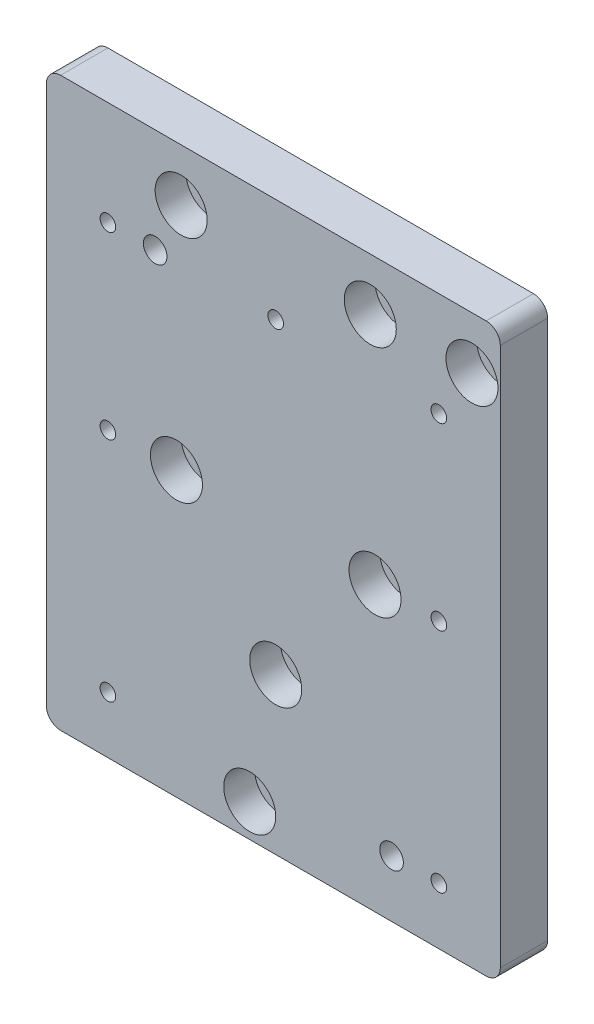
SolidWorks part; units mm, degrees
material "6061铝"
ref_plane "前视基准面" through (0, 0, 0) normal (0, 0, 1) x (1, 0, 0)
ref_plane "上视基准面" through (0, 0, 0) normal (0, 1, 0) x (1, 0, 0)
ref_plane "右视基准面" through (0, 0, 0) normal (1, 0, 0) x (0, 0, -1)
sketch "草图1" plane through (0, 0, 0) normal (0, 0, 1) x (1, 0, 0)
  line L1 (-48, 60) -> (48, 60)
  line L2 (-48, 60) -> (-48, -60)
  line L3 (-48, -60) -> (48, -60)
  line L4 (48, 60) -> (48, -60)
  line L5 (-48, 60) -> (48, -60) construction
  line L6 (-48, -60) -> (48, 60) construction
  point P0 (0, 0)
  dimension "D1" = 96
  dimension "D2" = 120
extrude "凸台-拉伸1" add sketch "草图1" along normal blind 10
hole_wizard "打孔尺寸(%根据)内六角圆柱头螺钉的类型2" positions "草图2" profile "草图4" counterbore size "M6" standard "GB" end condition through all
sketch "草图2" plane through (0, 0, 10) normal (0, 0, 1) x (1, 0, 0)
  point P0 (-19.5, 48.95)
  point P3 (20.5, 48.95)
  point P6 (42, 48.95)
  point P9 (21.5, -0.05)
  point P12 (-20.5, -0.05)
  point P15 (0.5, -27.05)
  point P18 (-5, -53.05)
sketch "草图4" plane through (-19.5, 48.95, 10) normal (1, 0, 0) x (0, -1, 0)
  line L0 (0, 0) -> (0, 10)
  line L1 (0, 10) -> (3.2, 10)
  line L3 (3.2, 10) -> (3.2, 6.5)
  line L4 (3.2, 6.5) -> (5.5, 6.5)
  line L5 (5.5, 6.5) -> (5.5, 0)
  line L7 (5.5, 0) -> (0, 0)
  line L11 (0, -6.35) -> (0, 107.95) construction
  dimension "通孔孔直径" = 6.4
  dimension "通孔孔深度" = 10
  dimension "柱形沉头孔直径" = 11
  dimension "柱形沉头孔深度" = 6.5
fillet "圆角1" radius 3 4 edges at (48, 60, 5) (-48, 60, 5) (-48, -60, 5) (48, -60, 5)
hole_wizard "M4 螺纹孔1" positions "草图5" profile "草图6" tap size "M4" standard "GB" end condition through all
sketch "草图5" plane through (0, 0, 10) normal (0, 0, 1) x (1, 0, 0)
  line L0 (0, 0) -> (0, -66.745) construction
  line L1 (-45, -60) -> (45, -60) construction
  line L2 (0.5, -27.05) -> (0.5, 29.2918) construction
  point P0 (-35, -48)
  point P6 (-35, 0)
  point P13 (35, 0)
  point P14 (35, -48)
  point P15 (-35, 38)
  point P23 (35, 38)
  point P26 (0.5, 38)
  point P47 (0, 0)
  point P48 (0, 0)
  dimension "D1" = 70
  dimension "D2" = 48
  dimension "D3" = 12
  dimension "D4" = 38
sketch "草图6" plane through (-35, -48, 10) normal (1, 0, 0) x (0, -1, 0)
  line L0 (0, 0) -> (0, 10)
  line L1 (0, 10) -> (1.65, 10)
  line L2 (1.65, 10) -> (1.65, 0)
  line L5 (1.65, 0) -> (0, 0)
  line L11 (0, -6.35) -> (0, 107.95) construction
  dimension "通孔螺纹孔钻头直径" = 3.3
  dimension "通孔螺纹孔钻头深度" = 10
cosmetic thread "孔螺蚊线1" parameters "D2"=4
cosmetic thread "孔螺蚊线2" parameters "D2"=4
cosmetic thread "孔螺蚊线3" parameters "D2"=4
cosmetic thread "孔螺蚊线4" parameters "D2"=4
cosmetic thread "孔螺蚊线5" parameters "D2"=4
cosmetic thread "孔螺蚊线6" parameters "D2"=4
cosmetic thread "孔螺蚊线7" parameters "D2"=4
sketch "草图7" plane through (0, 0, 10) normal (0, 0, 1) x (1, 0, 0)
  line L0 (-35, 38) -> (0.5, 38) construction
  line L1 (-35, -48) -> (36.65, -48) construction
  circle A0 centre (-25, 38) radius 2.5
  circle A1 centre (-35, 38) radius 1.65 construction
  circle A2 centre (35, -48) radius 1.65 construction
  circle A3 centre (25, -48) radius 2.5
  dimension "D1" = 5
  dimension "D2" = 10
  dimension "D3" = 5
  dimension "D4" = 10
extrude "切除-拉伸1" cut sketch "草图7" against normal blind 10
